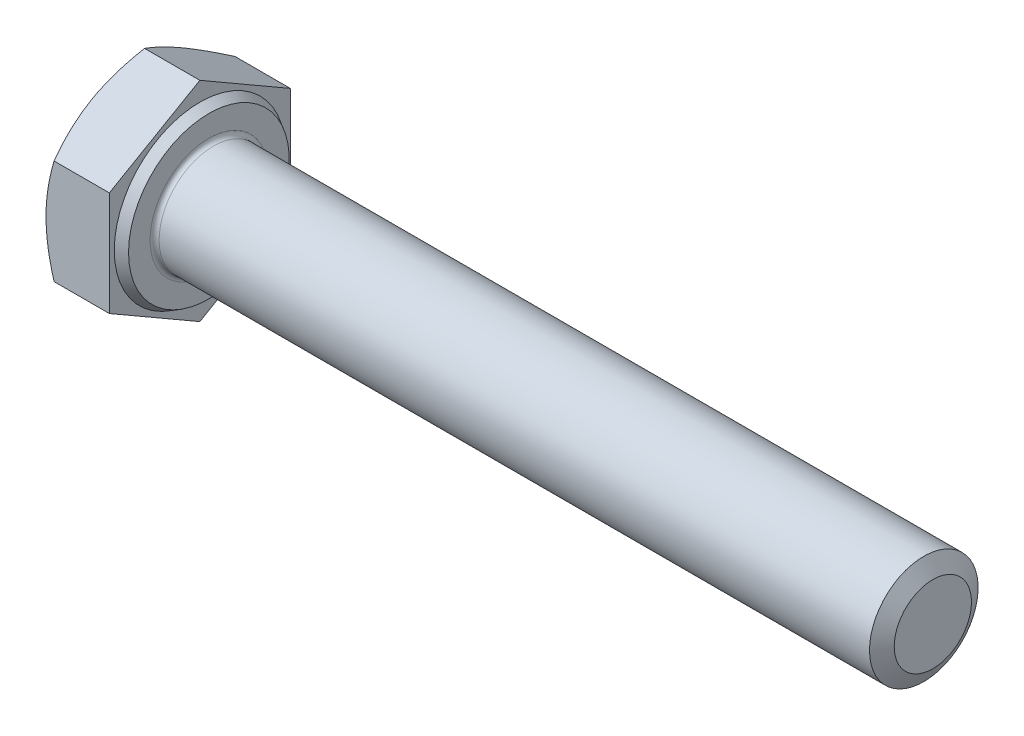
from build123d import *

# Parameters (mm, degrees)
EXTRUDE_390_DEPTH = 4
FILLET_1290_R     = 0.25


with BuildPart() as part:
    # 草图1 → Extrude 390 (new body)
    with BuildSketch(Plane(origin=(0, 0, 0), x_dir=(0, 0, -1), z_dir=(1, 0, 0))):
        Polygon((5, 2.886751346), (5, -2.886751346), (0, -5.773502692), (-5, -2.886751346), (-5, 2.886751346), (0, 5.773502692), align=None)
    extrude(amount=EXTRUDE_390_DEPTH)

    # 草图2 → 凸台-旋转1 (revolve)
    with BuildSketch(Plane.XY, mode=Mode.PRIVATE) as revolve_1_sk:
        Polygon((0, 0), (44, 0), (44, 2.134), (44, 3), (0, 3), align=None)
    revolve(revolve_1_sk.sketch.rotate(Axis((0, 0, 0), (1, 0, 0)), 90), axis=Axis((0, 0, 0), (1, 0, 0)))

    # 草图3 → 切除-旋转1 (revolve, cut)
    with BuildSketch(Plane.XY):
        Polygon((0, 5), (3.333333333, 10.773502692), (3.333333333, 15.773502692), (-10, 15.773502692), (-10, 5), align=None)
    revolve(axis=Axis((0, 0, 0), (1, 0, 0)), mode=Mode.SUBTRACT)

    # 草图4 → 切除-旋转3 (revolve, cut)
    with BuildSketch(Plane.XY, mode=Mode.PRIVATE) as cut_revolve_3_sk:
        Polygon((4, 4.44), (3.5, 4.728675135), (3.5, 5.773502692), (4, 5.773502692), align=None)
    revolve(cut_revolve_3_sk.sketch.rotate(Axis((0, 0, 0), (1, 0, 0)), 90), axis=Axis((0, 0, 0), (1, 0, 0)), mode=Mode.SUBTRACT)

    # Fillet 1290
    fillet_1290_edges = [part.edges().sort_by_distance(p)[0] for p in [
        (4, 0, -3),
    ]]
    fillet(fillet_1290_edges, radius=FILLET_1290_R)

    # 草图6 → 切除-旋转4 (revolve, cut)
    with BuildSketch(Plane.XY, mode=Mode.PRIVATE) as cut_revolve_4_sk:
        Polygon((43.5, 3), (44.5, 3), (44, 2.133974596), align=None)
    revolve(cut_revolve_4_sk.sketch.rotate(Axis((0, 0, 0), (1, 0, 0)), 90), axis=Axis((0, 0, 0), (1, 0, 0)), mode=Mode.SUBTRACT)


solid = part.part
